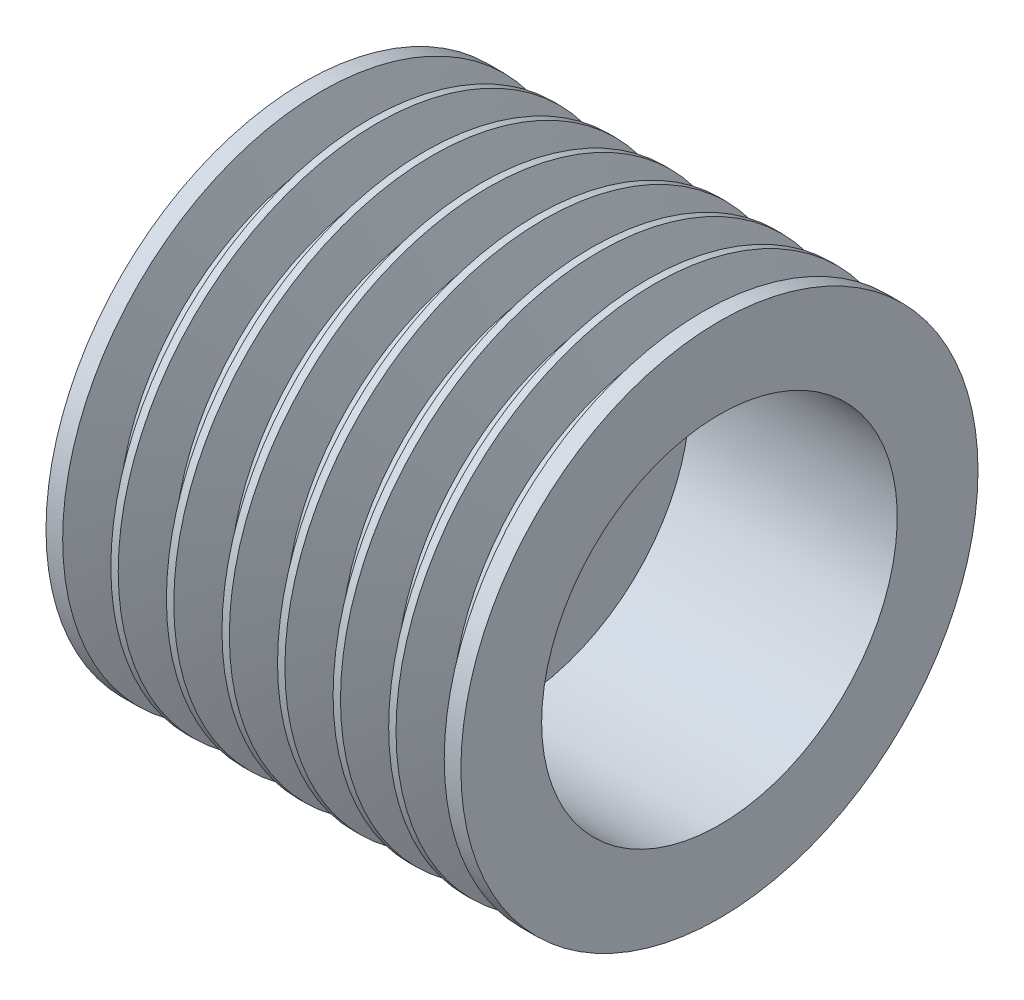
from build123d import *

# Parameters (mm, degrees)
SKETCH3_W          = 20
SKETCH3_H          = 43.741822135
CUT_EXTRUDE1_DEPTH = 374.22982196
LPATTERN1_COUNT    = 7
LPATTERN1_PITCH    = 37.5


with BuildPart() as part:
    # Sketch1 → Revolve1 (revolve)
    with BuildSketch(Plane.XY, mode=Mode.PRIVATE) as revolve1_sk:
        Polygon((0, 37.5), (-140, 37.5), (-140, 120), (-140, 174.5), (140, 174.5), (140, 120), (0, 120), align=None)
    revolve(revolve1_sk.sketch.rotate(Axis((0, 0, 0), (1, 0, 0)), 90), axis=Axis((0, 0, 0), (1, 0, 0)))

    # Sketch2 → Cut-Revolve1 (revolve, cut)
    with BuildSketch(Plane(origin=(0, 0, 0), x_dir=(1, 0, 0), z_dir=(0, 1, 0)), mode=Mode.PRIVATE) as cut_revolve1_sk:
        Polygon((-131.080105661, 181.63495756), (-119.501606075, 146), (-105.498393925, 146), (-93.919894339, 181.63495756), align=None)
    cut_revolve1 = revolve(cut_revolve1_sk.sketch.rotate(Axis((-238.897121458, 0, 0), (1, 0, 0)), 180), axis=Axis((-238.897121458, 0, 0), (1, 0, 0)), mode=Mode.SUBTRACT)

    # Sketch3 → Cut-Extrude1 (cut, through all)
    with BuildSketch(Plane.ZY.offset(140)):
        with Locations((0, 20.529088933)):
            Rectangle(SKETCH3_W, SKETCH3_H)
    extrude(amount=-CUT_EXTRUDE1_DEPTH, mode=Mode.SUBTRACT)

    # LPattern1: Cut-Revolve1 ×7
    with Locations(*[(i * LPATTERN1_PITCH, 0, 0) for i in range(1, LPATTERN1_COUNT)]):
        add(cut_revolve1, mode=Mode.SUBTRACT)


solid = part.part
